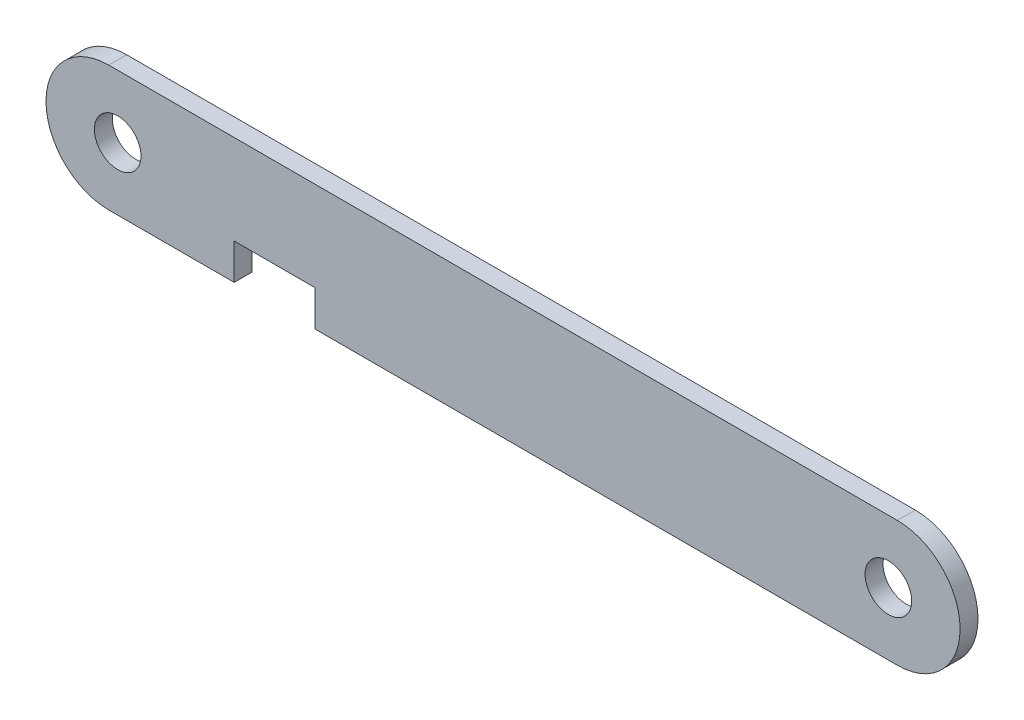
SolidWorks part; units mm, degrees
material "普通碳钢"
ref_plane "Front Plane" through (0, 0, 0) normal (0, 0, 1) x (1, 0, 0)
ref_plane "Top Plane" through (0, 0, 0) normal (0, 1, 0) x (1, 0, 0)
ref_plane "Right Plane" through (0, 0, 0) normal (1, 0, 0) x (0, 0, -1)
sketch "Sketch1" plane through (0, 0, 0) normal (0, 0, 1) x (1, 0, 0)
  line L0 (-30, -7) -> (-30, -3)
  line L1 (-44, 7) -> (44, 7)
  line L2 (-51, 7) -> (-51, -7) construction
  line L3 (-44, -7) -> (-30, -7)
  line L4 (51, 14.5063) -> (51, -36.9165) construction
  line L5 (-30, -3) -> (-21, -3)
  line L6 (-21, -3) -> (-21, -7)
  line L7 (-21, -7) -> (44, -7)
  arc A0 (-44, 7) -> (-44, -7) centre (-44, 0) ccw
  arc A1 (44, -7) -> (44, 7) centre (44, 0) ccw
  circle A2 centre (-43, 0) radius 2.6
  circle A3 centre (43, 0) radius 2.6
  dimension "D5" = 5.2
  dimension "D6" = 5.2
  dimension "D12" = 7
  dimension "D13" = 7
  dimension "D2" = 51
  dimension "D3" = 102
  dimension "D4" = 7
  dimension "D7" = 86
  dimension "D8" = 43
  dimension "D9" = 13
  dimension "D10" = 9
  dimension "D11" = 4
  dimension "D14" = 14
extrude "Extrude1" add sketch "Sketch1" along normal blind 2
